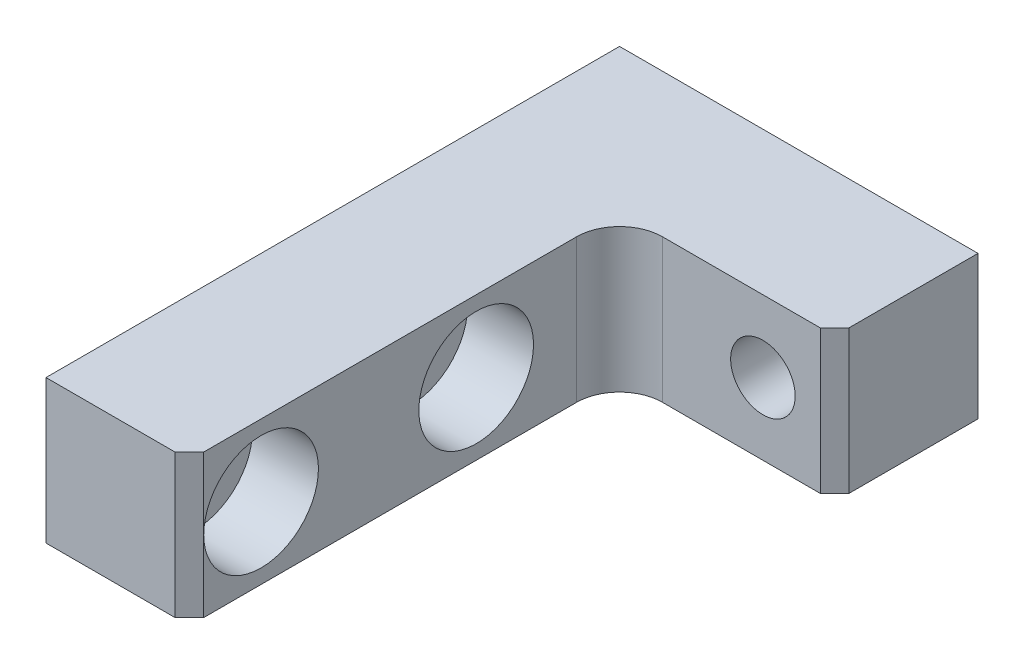
from build123d import *

# Parameters (mm, degrees)
SKETCH_1_W                = 25
SKETCH_1_H                = 40
EXTRUDE_1_DEPTH           = 5
CUT_EXTRUDE_1_DEPTH       = 10
CHAMFER_1_SIZE            = 1
HOLE_WIZARD_1_D           = 4.5
HOLE_WIZARD_1_CBORE_D     = 8
HOLE_WIZARD_1_CBORE_DEPTH = 4.6
HOLE_WIZARD_M4_1_D        = 4.5


with BuildPart() as part:
    # 草图1 → 凸台-拉伸1 (new, symmetric)
    with BuildSketch(Plane(origin=(0, 0, 0), x_dir=(1, 0, 0), z_dir=(0, 1, 0))):
        Rectangle(SKETCH_1_W, SKETCH_1_H)
    extrude(amount=EXTRUDE_1_DEPTH, both=True)

    # 草图2 → 切除-拉伸1 (cut)
    with BuildSketch(Plane(origin=(0, 5, 0), x_dir=(1, 0, 0), z_dir=(0, 1, 0))):
        with BuildLine():
            Line((12.5, -20), (-2.5, -20))
            Line((-2.5, -20), (-2.5, 7))
            ThreePointArc((-2.5, 7), (-1.621320344, 9.121320344), (0.5, 10))
            Line((0.5, 10), (12.5, 10))
            Line((12.5, 10), (12.5, -20))
        make_face()
    extrude(amount=-CUT_EXTRUDE_1_DEPTH, mode=Mode.SUBTRACT)

    # 倒角1
    chamfer_1_edges = [part.edges().sort_by_distance(p)[0] for p in [
        (-2.5, 0, 20),
        (12.5, 0, -10),
    ]]
    chamfer(chamfer_1_edges, length=CHAMFER_1_SIZE)

    # 打孔尺寸(%根据)内六角圆柱头螺钉的类型1 (through all)
    with Locations(Plane(origin=(-2.5, 0, 0), x_dir=(0, 0, -1), z_dir=(1, 0, 0))):
        with Locations((-15, 0), (0, 0)):
            CounterBoreHole(HOLE_WIZARD_1_D / 2, HOLE_WIZARD_1_CBORE_D / 2, HOLE_WIZARD_1_CBORE_DEPTH)

    # M4 间隙孔1 (through all)
    with Locations(Plane.XY.offset(-10)):
        with Locations((7.5, 0)):
            Hole(HOLE_WIZARD_M4_1_D / 2)


solid = part.part
